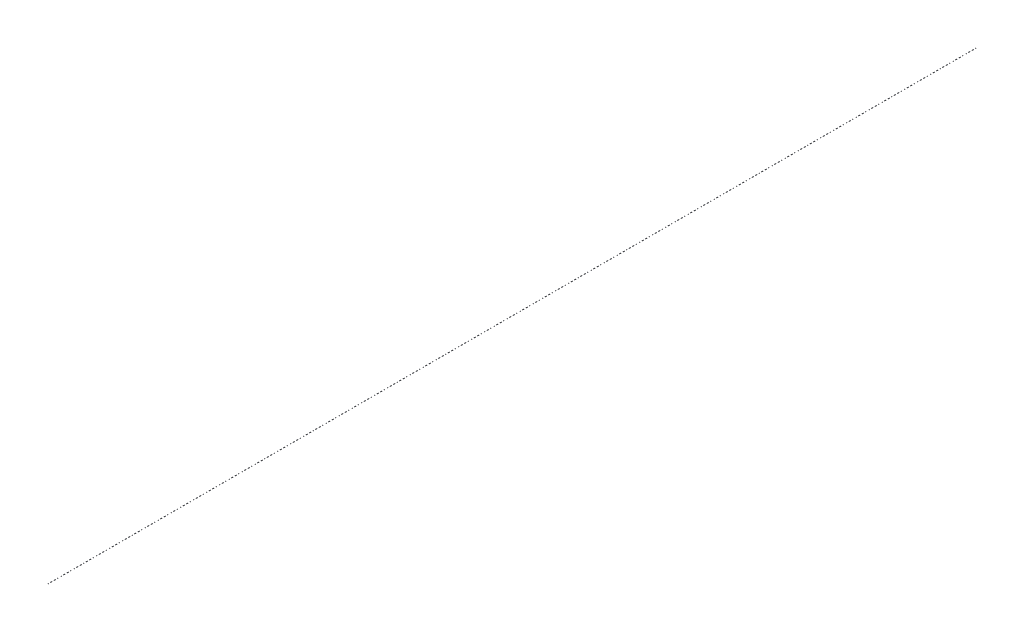
from build123d import *

# Parameters (mm, degrees)
SKETCH1_R           = 0.075
SKETCH1_R_2         = 0.0625
BOSS_EXTRUDE1_DEPTH = 1900


with BuildPart() as part:
    # Sketch1 → Boss-Extrude1 (new body)
    with BuildSketch(Plane.XY):
        Circle(SKETCH1_R)
        Circle(SKETCH1_R_2, mode=Mode.SUBTRACT)
    extrude(amount=BOSS_EXTRUDE1_DEPTH)


solid = part.part
